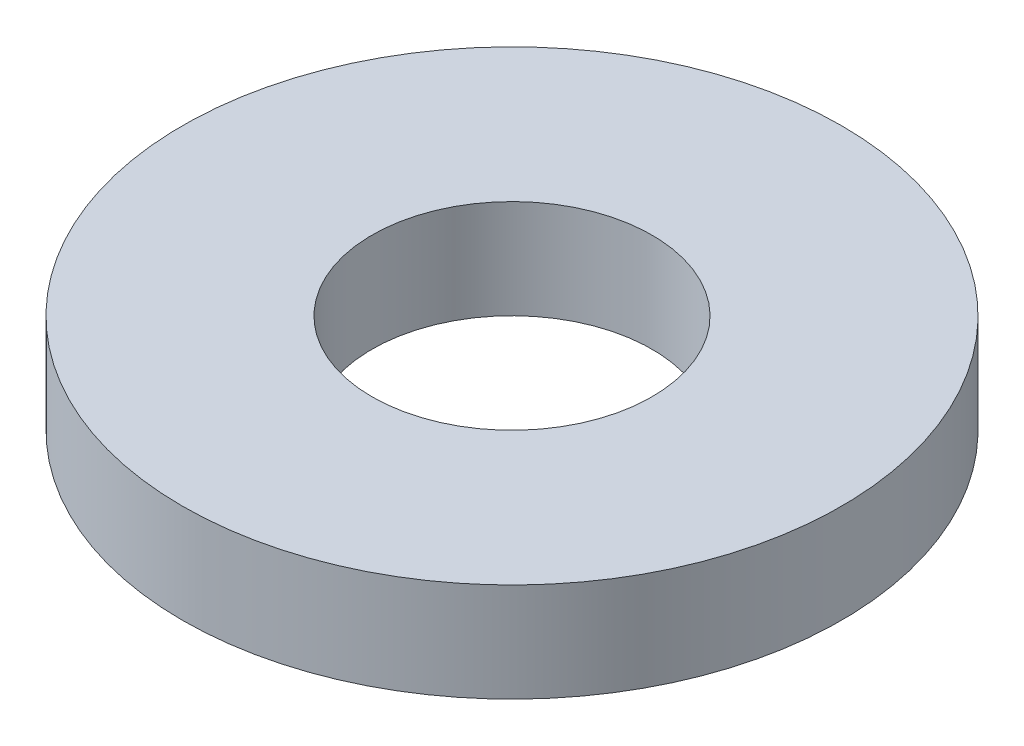
from build123d import *

# Parameters (mm, degrees)
SKETCH1_R           = 10
SKETCH1_R_2         = 4.25
BOSS_EXTRUDE1_DEPTH = 3


with BuildPart() as part:
    # Sketch1 → Boss-Extrude1 (new body)
    with BuildSketch(Plane(origin=(0, 0, 0), x_dir=(1, 0, 0), z_dir=(0, 1, 0))):
        with Locations(Location((0, 0, 0), (0, 0, 270))):
            Circle(SKETCH1_R)
        with Locations(Location((0, 0, 0), (0, 0, 270))):
            Circle(SKETCH1_R_2, mode=Mode.SUBTRACT)
    extrude(amount=BOSS_EXTRUDE1_DEPTH)


solid = part.part
